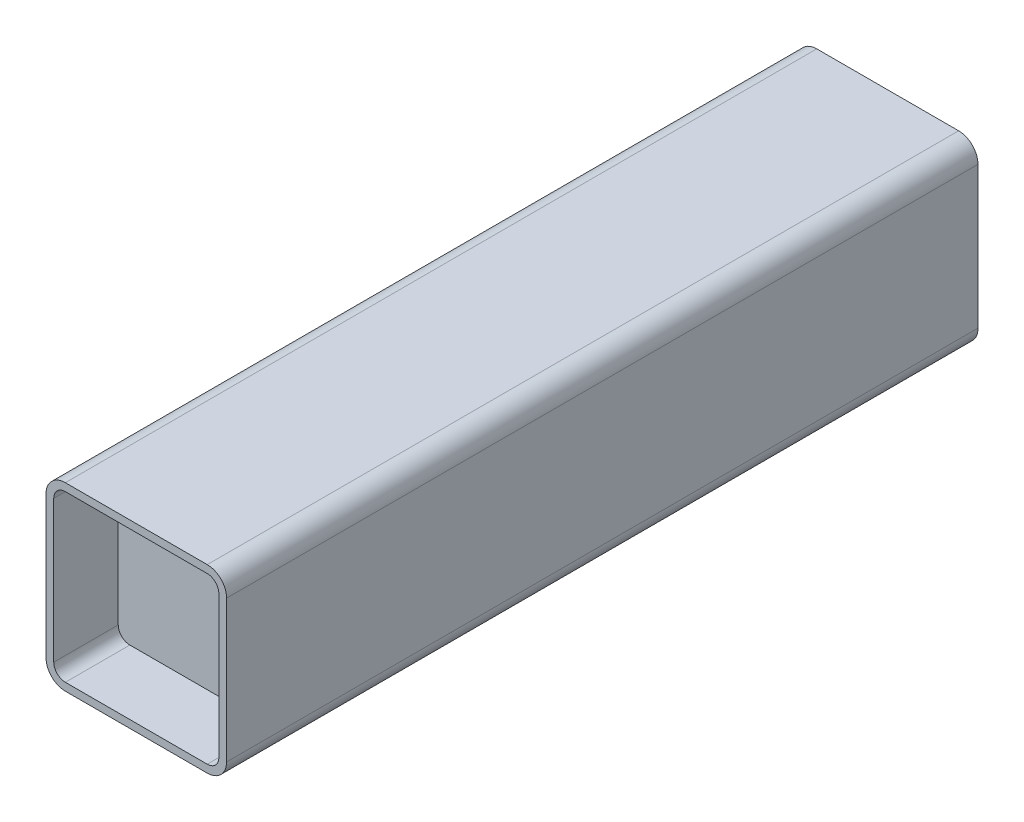
from build123d import *

# Parameters (mm, degrees)
EXTRUDE_1_DEPTH = 1165
EXTRUDE_START   = -110
EXTRUDE_2_DEPTH = 10
EXTRUDE_4_REACH = 1205.598
SKETCH_4_W      = 256
SKETCH_4_H      = 10


with BuildPart() as part:
    # 草图1 → 凸台-拉伸1 (new body)
    with BuildSketch(Plane.XY):
        with BuildLine():
            Line((-110, 140), (110, 140))
            ThreePointArc((110, 140), (131.213203436, 131.213203436), (140, 110))
            Line((140, 110), (140, -110))
            ThreePointArc((140, -110), (131.213203436, -131.213203436), (110, -140))
            Line((110, -140), (-110, -140))
            ThreePointArc((-110, -140), (-131.213203436, -131.213203436), (-140, -110))
            Line((-140, -110), (-140, 110))
            ThreePointArc((-140, 110), (-131.213203436, 131.213203436), (-110, 140))
        make_face()
        with BuildLine():
            Line((-110, 128), (110, 128))
            ThreePointArc((110, 128), (122.727922061, 122.727922061), (128, 110))
            Line((128, 110), (128, -110))
            ThreePointArc((128, -110), (122.727922061, -122.727922061), (110, -128))
            Line((110, -128), (-110, -128))
            ThreePointArc((-110, -128), (-122.727922061, -122.727922061), (-128, -110))
            Line((-128, -110), (-128, 110))
            ThreePointArc((-128, 110), (-122.727922061, 122.727922061), (-110, 128))
        make_face(mode=Mode.SUBTRACT)
    extrude(amount=EXTRUDE_1_DEPTH)

    # 草图2 → 凸台-拉伸2 (add)
    with BuildSketch(Plane.XY.offset(1165).offset(EXTRUDE_START)):
        with BuildLine():
            Line((128, -110), (128, 110))
            ThreePointArc((128, 110), (122.727922061, 122.727922061), (110, 128))
            Line((110, 128), (-110, 128))
            ThreePointArc((-110, 128), (-122.727922061, 122.727922061), (-128, 110))
            Line((-128, 110), (-128, -110))
            ThreePointArc((-128, -110), (-122.727922061, -122.727922061), (-110, -128))
            Line((-110, -128), (110, -128))
            ThreePointArc((110, -128), (122.727922061, -122.727922061), (128, -110))
        make_face()
    extrude_2 = extrude(amount=EXTRUDE_2_DEPTH)

    # 镜向1: 凸台-拉伸2 across plane
    add(extrude_2.mirror(Plane.XY.offset(582.5)))

    # 凸台-拉伸4: up to this face of the body (flat: up to its plane)
    extrude_4_end = Plane(part.part.faces().sort_by_distance((0, 128, 50))[0])
    # 草图4 → 凸台-拉伸4 (add, up to the picked face)
    with BuildSketch(Plane(origin=(0, -128, 0), x_dir=(1, 0, 0), z_dir=(0, 1, 0)), mode=Mode.PRIVATE) as extrude_4_sk1:
        with Locations((0, -740)):
            Rectangle(SKETCH_4_W, SKETCH_4_H)
    extrude_4_tool1 = split(extrude(extrude_4_sk1.sketch, amount=EXTRUDE_4_REACH, mode=Mode.PRIVATE), bisect_by=extrude_4_end, keep=Keep.BOTH, mode=Mode.PRIVATE)
    # 草图4 → 凸台-拉伸4 (add, up to the picked face)
    with BuildSketch(Plane(origin=(0, -128, 0), x_dir=(1, 0, 0), z_dir=(0, 1, 0)), mode=Mode.PRIVATE) as extrude_4_sk2:
        with Locations((0, -425)):
            Rectangle(SKETCH_4_W, SKETCH_4_H)
    extrude_4_tool2 = split(extrude(extrude_4_sk2.sketch, amount=EXTRUDE_4_REACH, mode=Mode.PRIVATE), bisect_by=extrude_4_end, keep=Keep.BOTH, mode=Mode.PRIVATE)
    add(extrude_4_tool1.solids().sort_by(Axis((0, -128, 740), (0, 1, 0)))[0])
    add(extrude_4_tool2.solids().sort_by(Axis((0, -128, 425), (0, 1, 0)))[0])


solid = part.part
